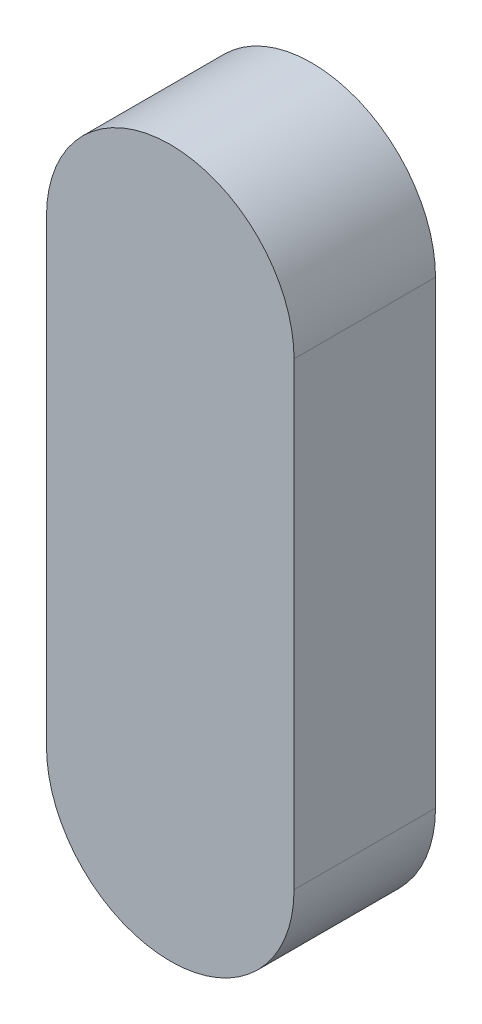
from build123d import *

# Parameters (mm, degrees)
EXTRUDE_1_DEPTH = 32


with BuildPart() as part:
    # 草图1 → 凸台-拉伸1 (new body)
    with BuildSketch(Plane.XY):
        with BuildLine():
            Line((0, 0), (0, 104))
            ThreePointArc((0, 104), (28, 132), (56, 104))
            Line((56, 104), (56, 0))
            ThreePointArc((56, 0), (28, -28), (0, 0))
        make_face()
    extrude(amount=EXTRUDE_1_DEPTH)


solid = part.part
